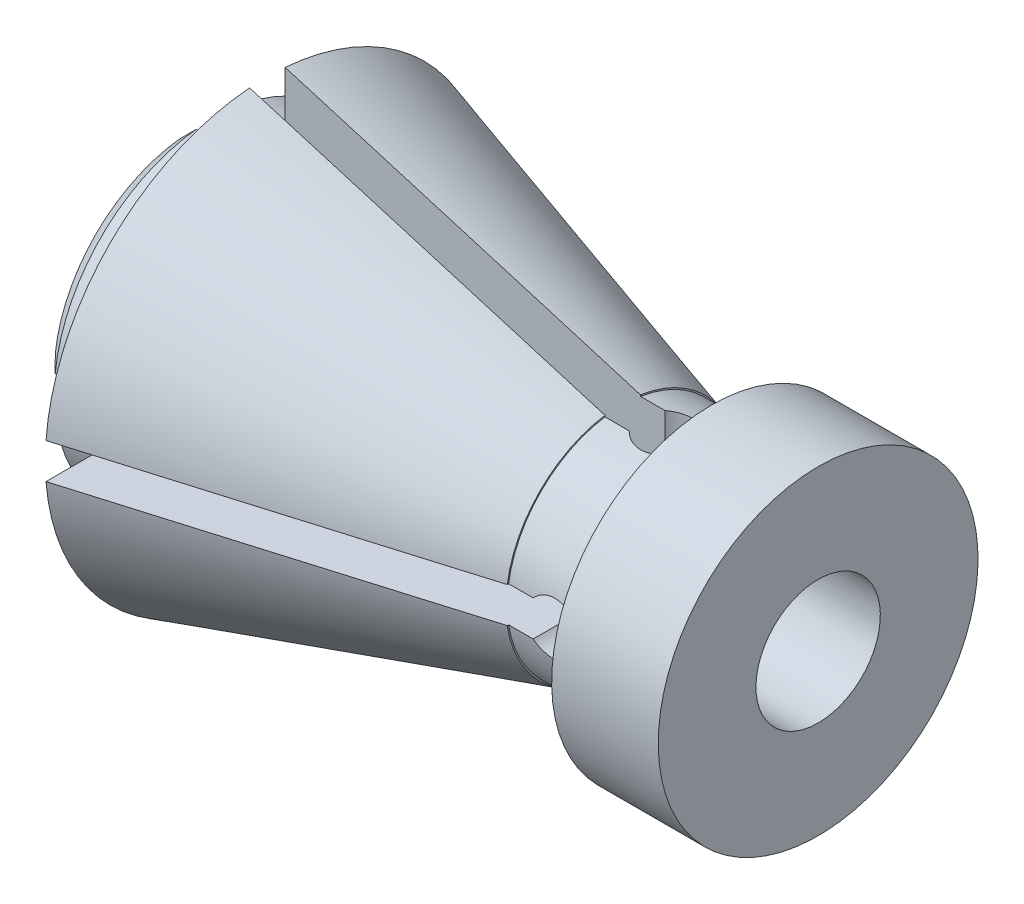
SolidWorks part; units mm, degrees
ref_plane "Front Plane" through (0, 0, 0) normal (0, 0, 1) x (1, 0, 0)
ref_plane "Top Plane" through (0, 0, 0) normal (0, 1, 0) x (1, 0, 0)
ref_plane "Right Plane" through (0, 0, 0) normal (1, 0, 0) x (0, 0, -1)
other "Configuration Table"
sketch "Sketch1" plane through (0, 0, 0) normal (0, 0, 1) x (1, 0, 0)
  line L0 (0, 0) -> (0, 9)
  line L1 (0, 9) -> (4, 9)
  line L2 (4, 9) -> (4, 12.5)
  line L3 (4, 12.5) -> (24, 6.5757)
  line L4 (24, 6.5757) -> (24, 6.5)
  line L5 (24, 6.5) -> (29, 6.5)
  line L6 (29, 6.5) -> (29, 9)
  line L7 (29, 9) -> (35, 9)
  line L8 (35, 9) -> (35, 0)
  line L9 (35, 0) -> (0, 0) construction
  line L10 (0, 0) -> (35, 0)
  dimension "D1" = 16.5
  dimension "D2" = 4
  dimension "D3" = 35
  dimension "D4" = 25
  dimension "D5" = 18
  dimension "D6" = 5
  dimension "D7" = 13
  dimension "D8" = 20
  dimension "D9" = 18
revolve "Revolve1" add sketch "Sketch1" angle 360 about L9
sketch "Sketch2" plane through (0, 0, 0) normal (-1, 0, 0) x (0, 0, 1)
  circle A0 centre (0, 0) radius 3.5
  dimension "D1" = 7
extrude "Cut-Extrude1" cut sketch "Sketch2" against normal through all
sketch "Sketch3" plane through (0, 0, 0) normal (0, 0, 1) x (1, 0, 0)
  line L0 (29, 6.5) -> (24, 6.5) construction
  circle A0 centre (26.5, 0) radius 1.5
  point P5 (26.5, 6.5)
  dimension "D1" = 3
extrude "Cut-Extrude2" cut sketch "Sketch3" against normal through all both and the other way through all
sketch "Sketch4" plane through (0, 0, 0) normal (0, 1, 0) x (1, 0, 0)
  line L0 (24, 6.5) -> (29, 6.5) construction
  circle A0 centre (26.5, 0) radius 1.5
  point P6 (26.5, 6.5)
  dimension "D1" = 3
extrude "Cut-Extrude3" cut sketch "Sketch4" against normal through all both and the other way through all
sketch "Sketch5" plane through (0, 0, 0) normal (0, 0, 1) x (1, 0, 0)
  line L1 (-25.382, -1) -> (25.382, -1)
  line L2 (-25.382, -1) -> (-25.382, 1)
  line L3 (-25.382, 1) -> (25.382, 1)
  line L4 (25.382, -1) -> (25.382, 1)
  line L5 (-25.382, -1) -> (25.382, 1) construction
  line L6 (-25.382, 1) -> (25.382, -1) construction
  circle A0 centre (26.5, 0) radius 1.5 construction
  point P0 (0, 0)
  dimension "D1" = 2
extrude "Cut-Extrude4" cut sketch "Sketch5" against normal through all both and the other way through all
sketch "Sketch6" plane through (0, 0, 0) normal (0, 1, 0) x (1, 0, 0)
  line L1 (-25.382, -1) -> (25.382, -1)
  line L2 (-25.382, -1) -> (-25.382, 1)
  line L3 (-25.382, 1) -> (25.382, 1)
  line L4 (25.382, -1) -> (25.382, 1)
  line L5 (-25.382, -1) -> (25.382, 1) construction
  line L6 (-25.382, 1) -> (25.382, -1) construction
  circle A0 centre (26.5, 0) radius 1.5 construction
  point P0 (0, 0)
  dimension "D1" = 2
extrude "Cut-Extrude5" cut sketch "Sketch6" against normal through all both and the other way through all
chamfer "Chamfer1" distance 1 angle 45 4 edges at (0, -6.364, 6.364) (0, -6.364, -6.364) (0, 6.364, -6.364) (0, 6.364, 6.364)
